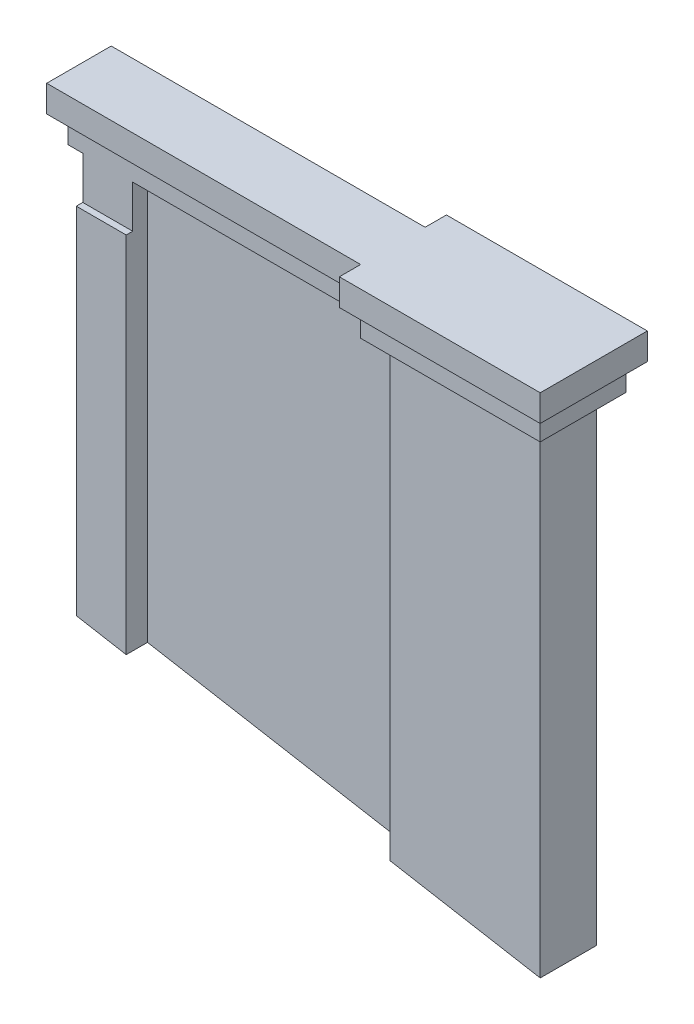
from build123d import *

# Parameters (mm, degrees)
BOSS_EXTRUDE1_DEPTH = 45
CUT_EXTRUDE1_DEPTH  = 63.865688575
BOSS_EXTRUDE2_DEPTH = 2.5
BOSS_EXTRUDE3_DEPTH = 2.5
SKETCH5_W           = 0.61
SKETCH5_H           = 4
CUT_EXTRUDE2_DEPTH  = 10


with BuildPart() as part:
    # Sketch1 → Boss-Extrude1 (new body)
    with BuildSketch(Plane(origin=(0, 0, 0), x_dir=(1, 0, 0), z_dir=(0, 1, 0))):
        Polygon((-43.58, 0), (-38.89, 0), (-38.89, 2), (-14.09, 2), (-14.09, 0), (0, 0), (0, 5.28), (-14.09, 5.28), (-14.09, 3.28), (-43.58, 3.28), align=None)
    extrude(amount=BOSS_EXTRUDE1_DEPTH)

    # Sketch2 → Cut-Extrude1 (cut, through all)
    with BuildSketch(Plane.XY):
        Polygon((0, 0), (-43.58, 0), (-43.58, 7.684329819), align=None)
    extrude(amount=-CUT_EXTRUDE1_DEPTH, mode=Mode.SUBTRACT)

    # Sketch3 → Boss-Extrude2 (add)
    with BuildSketch(Plane(origin=(0, 45, 0), x_dir=(1, 0, 0), z_dir=(0, 1, 0))):
        Polygon((-44.97, 4.67), (-44.97, 0.61), (-15.48, 0.61), (-15.48, -1.39), (1.39, -1.39), (1.39, 6.67), (-15.48, 6.67), (-15.48, 4.67), align=None)
    extrude(amount=BOSS_EXTRUDE2_DEPTH)

    # Sketch4 → Boss-Extrude3 (add)
    with BuildSketch(Plane(origin=(0, 47.5, 0), x_dir=(1, 0, 0), z_dir=(0, 1, 0))):
        Polygon((-45.97, 5.67), (-45.97, -0.39), (-16.48, -0.39), (-16.48, -2.39), (2.39, -2.39), (2.39, 7.67), (-16.48, 7.67), (-16.48, 5.67), align=None)
    extrude(amount=BOSS_EXTRUDE3_DEPTH)

    # Sketch5 → Cut-Extrude2 (cut)
    with BuildSketch(Plane.ZY.offset(43.58)):
        with Locations((-0.305, 43)):
            Rectangle(SKETCH5_W, SKETCH5_H)
    extrude(amount=-CUT_EXTRUDE2_DEPTH, mode=Mode.SUBTRACT)


solid = part.part
